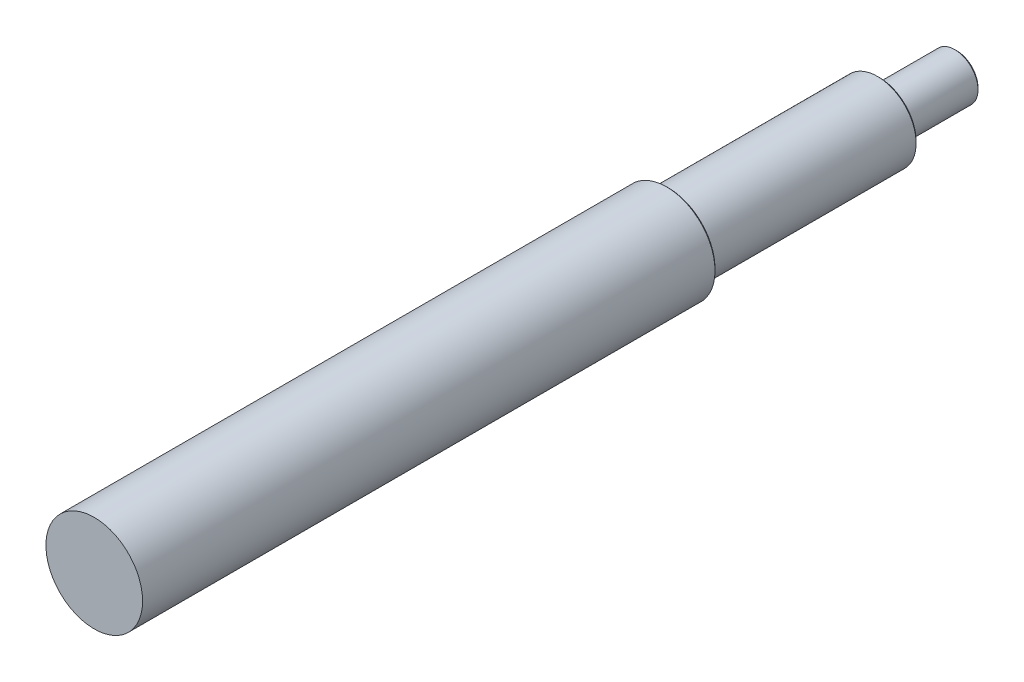
SolidWorks part; units mm, degrees
material "AISI 1045 钢，冷拔"
ref_plane "前视基准面" through (0, 0, 0) normal (0, 0, 1) x (1, 0, 0)
ref_plane "上视基准面" through (0, 0, 0) normal (0, 1, 0) x (1, 0, 0)
ref_plane "右视基准面" through (0, 0, 0) normal (1, 0, 0) x (0, 0, -1)
sketch "草图1" plane through (0, 0, 0) normal (0, 0, 1) x (1, 0, 0)
  circle A0 centre (0, 0) radius 25
  dimension "D1" = 50
extrude "凸台-拉伸1" add sketch "草图1" along normal blind 100 and the other way blind 346
ref_plane "基准面1" through (0, 0, -306) normal (0, 0, -1) x (-1, 0, 0)
sketch "草图2" plane through (0, 0, -306) normal (0, 0, -1) x (-1, 0, 0)
  circle A0 centre (0, 0) radius 25
  circle A1 centre (0, 0) radius 20
extrude "切除-拉伸1" cut sketch "草图2" against normal blind 109
sketch "草图3" plane through (0, 0, -346) normal (0, 0, -1) x (-1, 0, 0)
  circle A0 centre (0, 0) radius 25
  circle A1 centre (0, 0) radius 12
extrude "切除-拉伸2" cut sketch "草图3" against normal blind 40
cosmetic thread "装饰螺纹线1" parameters "D2"=22
chamfer "倒角1" distance 1 angle 45 3 edges at (-12, 0, -346) (-20, 0, -306) (-25, 0, -197)
